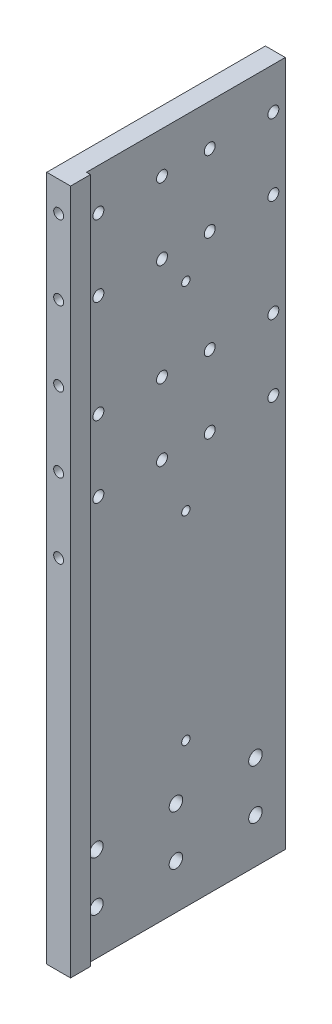
from build123d import *

# Parameters (mm, degrees)
SKETCH_1_W                   = 110
SKETCH_1_H                   = 345
EXTRUDE_1_DEPTH              = 6
SKETCH_2_W                   = 100
SKETCH_2_H                   = 345
CUT_EXTRUDE_1_DEPTH          = 2
HOLE_WIZARD_M5_1_D           = 5.5
HOLE_WIZARD_M5_1_CBORE_D     = 10
HOLE_WIZARD_M5_1_CBORE_DEPTH = 5.4
HOLE_WIZARD_M8_1_D           = 6.8
HOLE_WIZARD_M6_1_D           = 5
HOLE_WIZARD_M6_1_DEPTH       = 15
HOLE_WIZARD_M6_1_TIP         = 1.502151548
HOLE_WIZARD_M5_1_2_D         = 4.2


with BuildPart() as part:
    # 草图1 → 凸台-拉伸1 (new, symmetric)
    with BuildSketch(Plane(origin=(0, 0, 0), x_dir=(0, 0, -1), z_dir=(1, 0, 0))):
        Rectangle(SKETCH_1_W, SKETCH_1_H)
    extrude(amount=EXTRUDE_1_DEPTH, both=True)

    # 草图2 → 切除-拉伸1 (cut)
    with BuildSketch(Plane(origin=(6, 0, 0), x_dir=(0, 0, -1), z_dir=(1, 0, 0))):
        with Locations((5, 0)):
            Rectangle(SKETCH_2_W, SKETCH_2_H)
    extrude(amount=-CUT_EXTRUDE_1_DEPTH, mode=Mode.SUBTRACT)

    # Hole Wizard M5 _1 (through all)
    with Locations(Plane.ZY.offset(6)):
        with Locations((-49, 151.75), (-17, 151.75), (7, 151.75), (39, 151.75), (39, 115.75), (7, 115.75), (-17, 115.75), (-49, 115.75), (-49, 64.25), (-49, 28.25), (-17, 64.25), (-17, 28.25), (7, 64.25), (7, 28.25), (39, 64.25), (39, 28.25)):
            CounterBoreHole(HOLE_WIZARD_M5_1_D / 2, HOLE_WIZARD_M5_1_CBORE_D / 2, HOLE_WIZARD_M5_1_CBORE_DEPTH)

    # M8 螺纹孔1 (through all)
    with Locations(Plane.ZY.offset(6)):
        with Locations((-40, -125), (-40, -150), (0, -125), (0, -150), (40, -125), (40, -150)):
            Hole(HOLE_WIZARD_M8_1_D / 2)

    # M6 螺纹孔1
    with Locations(Plane.XY.offset(55)):
        with Locations((0, 7.5), (0, 45), (0, 82.5), (0, 120), (0, 157.5)):
            Hole(HOLE_WIZARD_M6_1_D / 2, depth=HOLE_WIZARD_M6_1_DEPTH)
            with Locations((0, 0, -(HOLE_WIZARD_M6_1_DEPTH + HOLE_WIZARD_M6_1_TIP / 2))):  # 118° drill point
                Cone(0, HOLE_WIZARD_M6_1_D / 2, HOLE_WIZARD_M6_1_TIP, mode=Mode.SUBTRACT)

    # Hole Wizard M5 _1 2 (through all)
    with Locations(Plane.ZY.offset(6)):
        with Locations((-5, 185), (-5, 100), (-5, 0), (-5, -100)):
            Hole(HOLE_WIZARD_M5_1_2_D / 2)


solid = part.part
